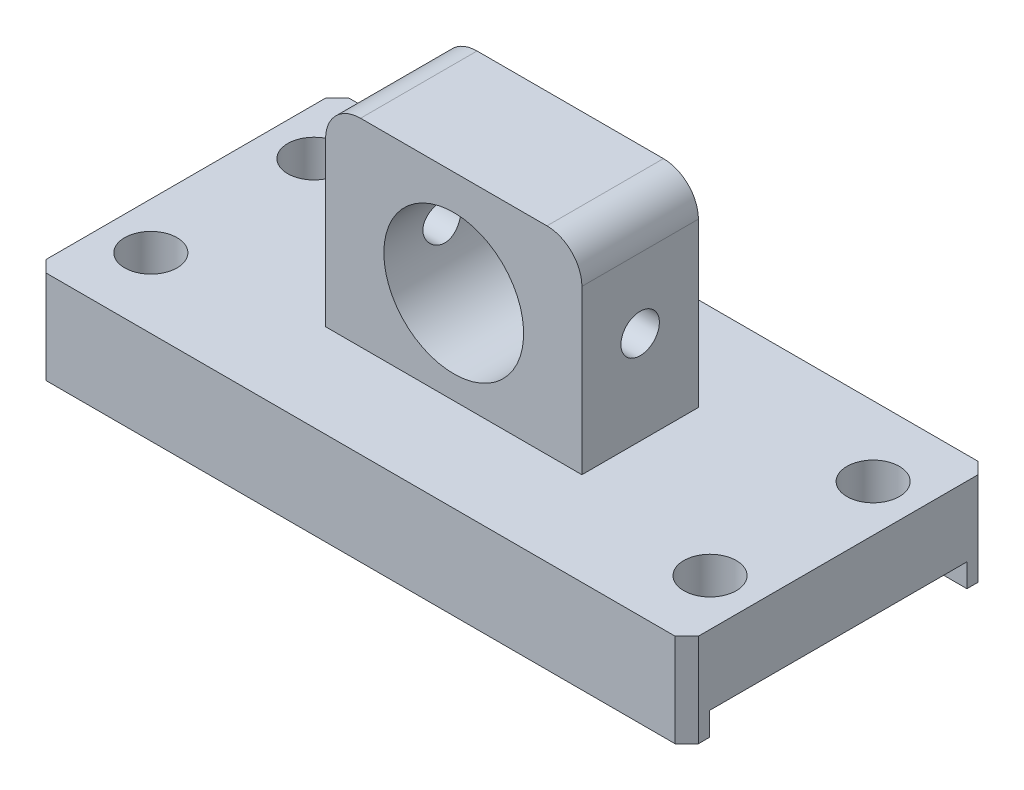
SolidWorks part; units mm, degrees
ref_plane "前视基准面" through (0, 0, 0) normal (0, 0, 1) x (1, 0, 0)
ref_plane "上视基准面" through (0, 0, 0) normal (0, 1, 0) x (1, 0, 0)
ref_plane "右视基准面" through (0, 0, 0) normal (1, 0, 0) x (0, 0, -1)
sketch "草图1" plane through (0, 0, 0) normal (0, 1, 0) x (1, 0, 0)
  line L1 (-28, 13) -> (28, 13)
  line L2 (-28, 13) -> (-28, -13)
  line L3 (-28, -13) -> (28, -13)
  line L4 (28, 13) -> (28, -13)
  line L5 (-28, 13) -> (28, -13) construction
  line L6 (-28, -13) -> (28, 13) construction
  point P0 (0, 0)
  dimension "D1" = 56
  dimension "D2" = 26
extrude "凸台-拉伸1" add sketch "草图1" along normal blind 8
sketch "草图2" plane through (0, 0, 0) normal (0, -1, 0) x (1, 0, 0)
  line L1 (-35.0157, 11.05) -> (35.0157, 11.05)
  line L2 (-35.0157, 11.05) -> (-35.0157, -11.05)
  line L3 (-35.0157, -11.05) -> (35.0157, -11.05)
  line L4 (35.0157, 11.05) -> (35.0157, -11.05)
  line L5 (-35.0157, 11.05) -> (35.0157, -11.05) construction
  line L6 (-35.0157, -11.05) -> (35.0157, 11.05) construction
  point P0 (0, 0)
  dimension "D1" = 22.1
extrude "切除-拉伸1" cut sketch "草图2" against normal blind 2
sketch "草图3" plane through (0, 8, 0) normal (0, 1, 0) x (1, 0, 0)
  line L1 (-11, 5) -> (11, 5)
  line L2 (-11, 5) -> (-11, -5)
  line L3 (-11, -5) -> (11, -5)
  line L4 (11, 5) -> (11, -5)
  line L5 (-11, 5) -> (11, -5) construction
  line L6 (-11, -5) -> (11, 5) construction
  point P0 (0, 0)
  dimension "D1" = 10
  dimension "D2" = 22
extrude "凸台-拉伸2" add sketch "草图3" along normal blind 17
sketch "草图4" plane through (0, 0, -13) normal (0, 0, -1) x (-1, 0, 0)
  line L0 (0, 16) -> (0, 0) construction
  circle A0 centre (0, 16) radius 6
  dimension "D2" = 12
  dimension "D1" = 16
extrude "切除-拉伸2" cut sketch "草图4" against normal through all
sketch "草图5" plane through (0, 0, -13) normal (0, 0, -1) x (-1, 0, 0)
  line L1 (-26.9868, 22) -> (0, 22)
  line L2 (-26.9868, 22) -> (-26.9868, 20)
  line L3 (-26.9868, 20) -> (0, 20)
  line L4 (0, 22) -> (0, 20)
  line L5 (-26.9868, 22) -> (0, 20) construction
  line L6 (-26.9868, 20) -> (0, 22) construction
  circle A0 centre (0, 16) radius 6 construction
  point P0 (-13.4934, 21)
  dimension "D2" = 2
extrude "切除-拉伸3" [suppressed] cut sketch "草图5" against normal through all
fillet "圆角1" [suppressed] radius 8
hole_wizard "Ø4.5 (4.5) 直径孔1" positions "草图7" profile "草图6" hole size "Ø4.5" standard "GB" end condition through all
sketch "草图7" plane through (0, 8, 0) normal (0, 1, 0) x (1, 0, 0)
  line L0 (-24, 7) -> (24, 7) construction
  line L1 (24, 7) -> (24, -7) construction
  line L4 (24, 0) -> (0, 0) construction
  line L5 (0, 0) -> (0, 7) construction
  point P0 (-24, 7)
  point P2 (-24, -7)
  point P4 (24, 7)
  point P6 (24, -7)
  dimension "D1" = 14
  dimension "D2" = 48
sketch "草图6" plane through (-24, 8, -7) normal (1, 0, 0) x (0, 0, 1)
  line L0 (0, 0) -> (0, 8)
  line L1 (0, 8) -> (2.25, 8)
  line L2 (2.25, 8) -> (2.25, 0)
  line L5 (2.25, 0) -> (0, 0)
  line L11 (0, -6.35) -> (0, 107.95) construction
  dimension "通孔孔直径" = 4.5
  dimension "通孔孔深度" = 8
fillet "圆角2" radius 3 2 edges at (-11, 25, 0) (11, 25, 0)
hole_wizard "M4 螺纹孔1" positions "草图9" profile "草图8" tap size "M4" standard "GB" end condition through all
sketch "草图9" plane through (11, 0, 0) normal (1, 0, 0) x (0, 0, -1)
  line L0 (-5, 25) -> (5, 25) construction
  line L1 (5, 22) -> (5, 8) construction
  point P0 (0, 16)
  dimension "D1" = 9
  dimension "D2" = 5
sketch "草图8" plane through (11, 16, 0) normal (0, 1, 0) x (0, 0, -1)
  line L0 (0, 0) -> (0, 39)
  line L1 (0, 39) -> (1.65, 39)
  line L2 (1.65, 39) -> (1.65, 0)
  line L5 (1.65, 0) -> (0, 0)
  line L11 (0, -6.35) -> (0, 107.95) construction
  dimension "通孔螺纹孔钻头直径" = 3.3
  dimension "通孔螺纹孔钻头深度" = 39
cosmetic thread "孔螺蚊线1" parameters "D2"=4
sketch "草图10" plane through (0, 8, 0) normal (0, 1, 0) x (1, 0, 0)
  line L1 (-28, -13) -> (28, -13) construction
  circle A0 centre (0, -18) radius 8
  dimension "D1" = 16
  dimension "D2" = 5
extrude "切除-拉伸6" [suppressed] cut sketch "草图10" against normal through all
chamfer "倒角1" distance 1 angle 45 4 edges at (-28, 4, -13) (-28, 4, 13) (28, 4, 13) (28, 4, -13)
